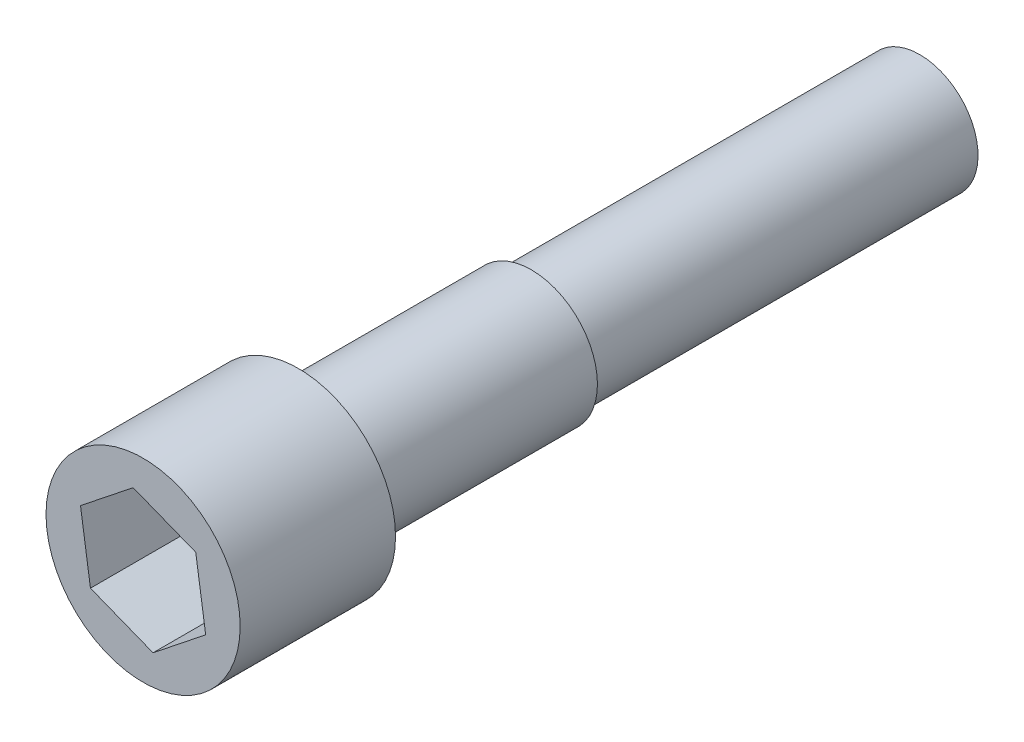
SolidWorks part; units mm, degrees
ref_plane "前视基准面" through (0, 0, 0) normal (0, 0, 1) x (1, 0, 0)
ref_plane "上视基准面" through (0, 0, 0) normal (0, 1, 0) x (1, 0, 0)
ref_plane "右视基准面" through (0, 0, 0) normal (1, 0, 0) x (0, 0, -1)
sketch "草图1" plane through (0, 0, 0) normal (0, 0, 1) x (1, 0, 0)
  circle A0 centre (0, -6) radius 1.7
  dimension "D1" = 3.4
extrude "凸台-拉伸1" add sketch "草图1" against normal up to surface (5.9985 mm away)
sketch "草图2" plane through (0, 0, -5.9985) normal (0, 0, -1) x (-1, 0, 0)
  circle A0 centre (0, -6) radius 1.5
  dimension "D1" = 3
extrude "凸台-拉伸2" add sketch "草图2" along normal up to surface (10 mm away)
sketch "草图3" plane through (0, 0, 0) normal (0, 0, 1) x (1, 0, 0)
  circle A0 centre (0, -6) radius 2.5
  dimension "D1" = 5
extrude "凸台-拉伸3" add sketch "草图3" along normal blind 4
sketch "草图4" plane through (0, 0, 4) normal (0, 0, 1) x (1, 0, 0)
  line L1 (1.3556, -4.9218) -> (-0.256, -4.287)
  line L2 (-0.256, -4.287) -> (-1.6115, -5.3651)
  line L3 (-1.6115, -5.3651) -> (-1.3556, -7.0782)
  line L4 (-1.3556, -7.0782) -> (0.256, -7.713)
  line L5 (0.256, -7.713) -> (1.6115, -6.6349)
  line L6 (1.6115, -6.6349) -> (1.3556, -4.9218)
  circle A0 centre (0, -6) radius 1.5 construction
  dimension "D1" = 3
extrude "切除-拉伸1" cut sketch "草图4" against normal blind 3
sketch "草图5" plane through (0, 0, 0) normal (0, 0, -1) x (-1, 0, 0)
  point P0 (-0.0669, -6)
